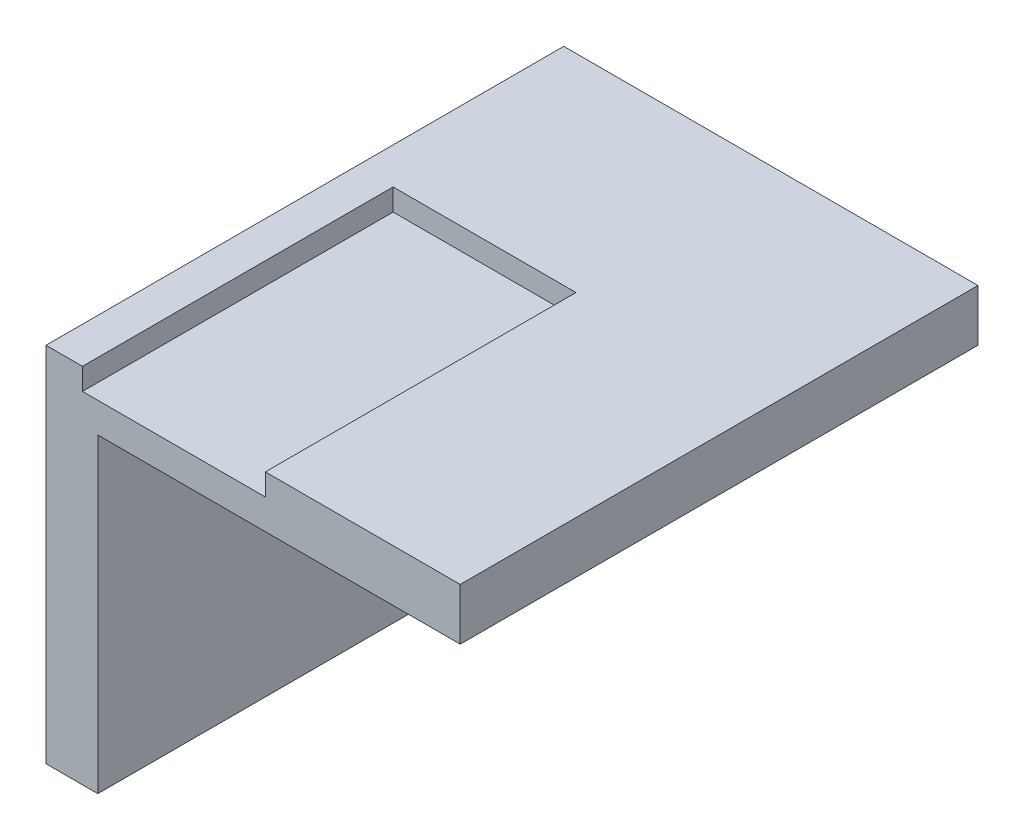
from build123d import *

# Parameters (mm, degrees)
EXTRUDE_1_DEPTH     = 100
SKETCH_2_W          = 35.317953013
SKETCH_2_H          = 4.2
CUT_EXTRUDE_1_DEPTH = 60


with BuildPart() as part:
    # 草图1 → 凸台-拉伸1 (new body)
    with BuildSketch(Plane.XY):
        Polygon((-37.5, 32.788461538), (42.5, 32.788461538), (42.5, 22.788461538), (-27.5, 22.788461538), (-27.5, -37.211538462), (-37.5, -37.211538462), align=None)
    extrude(amount=EXTRUDE_1_DEPTH)

    # 草图2 → 切除-拉伸1 (cut)
    with BuildSketch(Plane.XY.offset(100)):
        with Locations((-12.799064643, 30.688461538)):
            Rectangle(SKETCH_2_W, SKETCH_2_H)
    extrude(amount=-CUT_EXTRUDE_1_DEPTH, mode=Mode.SUBTRACT)


solid = part.part
